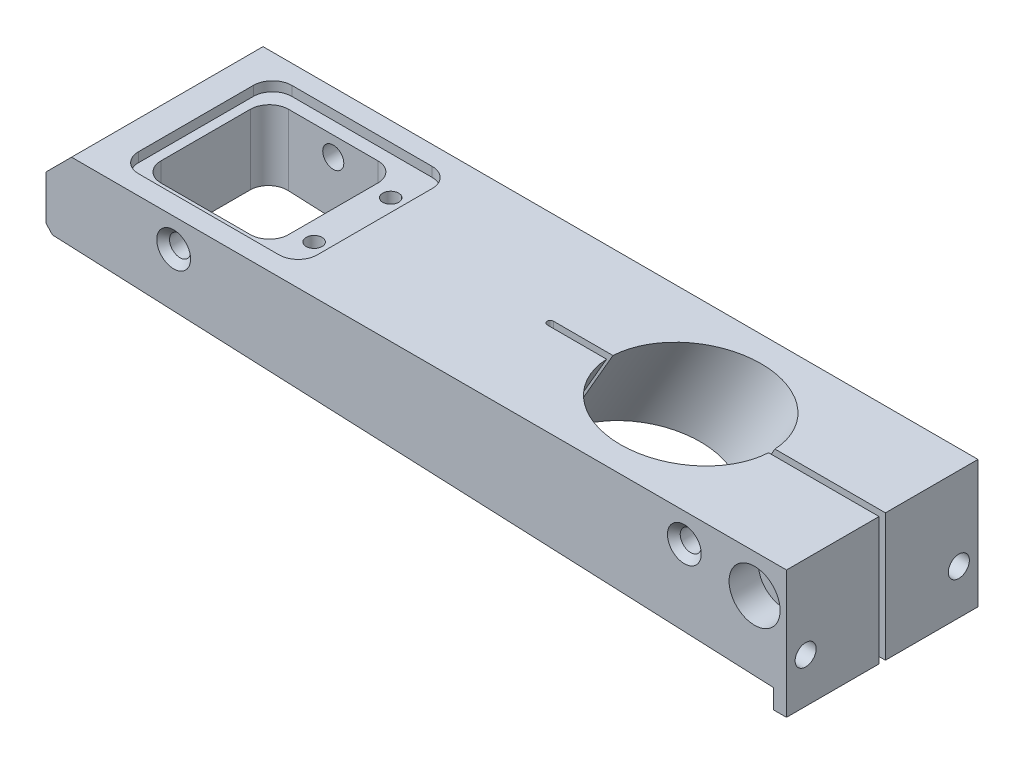
from build123d import *

# Parameters (mm, degrees)
SKETCH1_W                                            = 116
SKETCH1_H                                            = 30
BOSS_EXTRUDE1_DEPTH                                  = 10
CUT_EXTRUDE2_DEPTH                                   = 64.158530699
HOLE_SIZE_PER_SOCKET_HEAD_CAP_SCREW_TYPE_D           = 4.5
HOLE_SIZE_PER_SOCKET_HEAD_CAP_SCREW_TYPE_DEPTH       = 14.5
HOLE_SIZE_PER_SOCKET_HEAD_CAP_SCREW_TYPE_CBORE_D     = 8
HOLE_SIZE_PER_SOCKET_HEAD_CAP_SCREW_TYPE_CBORE_DEPTH = 4.6
M4_TAPPED_HOLE1_D                                    = 3.3
F_5_0_5_DIAMETER_HOLE1_D                             = 5
F_5_0_5_DIAMETER_HOLE1_DEPTH                         = 7
F_5_0_5_DIAMETER_HOLE1_TIP                           = 1.502151548
M4_TAPPED_HOLE2_AT_2_COUNT                           = 2
M4_TAPPED_HOLE2_AT_2_PITCH                           = 80
CHAMFER1_SIZE                                        = 4
M4_TAPPED_HOLE3_D                                    = 3.3
M4_TAPPED_HOLE3_DEPTH                                = 10.1
M4_TAPPED_HOLE3_TIP                                  = 0.991420021
CUT_EXTRUDE3_DEPTH                                   = 67.060578275
SKETCH18_W                                           = 20
SKETCH18_H                                           = 20
CUT_EXTRUDE4_DEPTH                                   = 64.158530699
SKETCH19_W                                           = 28
SKETCH19_H                                           = 24
CUT_EXTRUDE5_DEPTH                                   = 1.5
FILLET1_R                                            = 3
M3_TAPPED_HOLE1_D                                    = 2.5
M3_TAPPED_HOLE1_DEPTH                                = 7.5
M3_TAPPED_HOLE1_TIP                                  = 0.751075774
CHAMFER2_SIZE                                        = 1
CHAMFER2_SIZE2                                       = 1.04665043
CHAMFER3_SIZE                                        = 1


with BuildPart() as part:
    # Sketch1 → Boss-Extrude1 (new, symmetric)
    with BuildSketch(Plane(origin=(0, 0, 0), x_dir=(1, 0, 0), z_dir=(0, 1, 0))):
        Rectangle(SKETCH1_W, SKETCH1_H)
    extrude(amount=BOSS_EXTRUDE1_DEPTH, both=True)

    # Sketch3 → Cut-Revolve1 (revolve, cut)
    with BuildSketch(Plane.XY):
        Polygon((-39.473720558, -128.867912183), (58.526279442, 40.873066959), (49, 46.373066959), (-49, -123.367912183), align=None)
    revolve(axis=Axis((28, 10, 0), (-0.5000000000000041, -0.8660254037844363, 0)), mode=Mode.SUBTRACT)

    # Sketch4 → Cut-Extrude2 (cut, through all)
    with BuildSketch(Plane(origin=(0, 10, 0), x_dir=(1, 0, 0), z_dir=(0, 1, 0))):
        with BuildLine():
            Line((6, 0.5), (58, 0.5))
            Line((58, 0.5), (58, -0.5))
            Line((58, -0.5), (6, -0.5))
            ThreePointArc((6, -0.5), (5.5, 0), (6, 0.5))
        make_face()
    extrude(amount=-CUT_EXTRUDE2_DEPTH, mode=Mode.SUBTRACT)

    # Hole size per socket head cap screw type1
    with Locations(Plane.XY.offset(15)):
        with Locations((53, 4)):
            CounterBoreHole(HOLE_SIZE_PER_SOCKET_HEAD_CAP_SCREW_TYPE_D / 2, HOLE_SIZE_PER_SOCKET_HEAD_CAP_SCREW_TYPE_CBORE_D / 2, HOLE_SIZE_PER_SOCKET_HEAD_CAP_SCREW_TYPE_CBORE_DEPTH, depth=HOLE_SIZE_PER_SOCKET_HEAD_CAP_SCREW_TYPE_DEPTH)

    # M4 Tapped Hole1 (through all)
    with Locations(Plane.XY.offset(-0.5)):
        with Locations((53, 4)):
            Hole(M4_TAPPED_HOLE1_D / 2)

    # Ø5.0 (5) Diameter Hole1
    with Locations(Plane(origin=(0, 0, -15), x_dir=(-1, 0, 0), z_dir=(0, 0, -1))):
        with Locations((-53, 4)):
            Hole(F_5_0_5_DIAMETER_HOLE1_D / 2, depth=F_5_0_5_DIAMETER_HOLE1_DEPTH)
            with Locations((0, 0, -(F_5_0_5_DIAMETER_HOLE1_DEPTH + F_5_0_5_DIAMETER_HOLE1_TIP / 2))):  # 118° drill point
                Cone(0, F_5_0_5_DIAMETER_HOLE1_D / 2, F_5_0_5_DIAMETER_HOLE1_TIP, mode=Mode.SUBTRACT)

    # Sketch11 → M4 Tapped Hole2 (revolve, cut)
    with BuildSketch(Plane(origin=(-38, 5.5, 15), x_dir=(0, -1, 0), z_dir=(1, 0, 0))):
        Polygon((0, 0), (0, 11.091420021), (1.65, 10.1), (1.65, 0), align=None)
    m4_tapped_hole2 = revolve(axis=Axis((-38, 5.5, 21.35), (0, 0, -1)), mode=Mode.SUBTRACT)

    # M4 Tapped Hole2 at 2: M4 Tapped Hole2 ×2
    with Locations(*[(i * M4_TAPPED_HOLE2_AT_2_PITCH, 0, 0) for i in range(1, M4_TAPPED_HOLE2_AT_2_COUNT)]):
        add(m4_tapped_hole2, mode=Mode.SUBTRACT)

    # Mirror1: M4 Tapped Hole2 across plane
    add(m4_tapped_hole2.mirror(Plane.XY), mode=Mode.SUBTRACT)

    # Mirror1 copy 1 sketch → Mirror1 copy 1 (revolve, cut)
    with BuildSketch(Plane(origin=(42, 5.5, -15), x_dir=(0, -1, 0), z_dir=(1, 0, 0))):
        Polygon((0, 0), (0, -11.091420021), (1.65, -10.1), (1.65, 0), align=None)
    revolve(axis=Axis((42, 5.5, -21.35), (0, 0, -1)), mode=Mode.SUBTRACT)

    # Chamfer1
    chamfer1_edges = [part.edges().sort_by_distance(p)[0] for p in [
        (-58, 10, 0),
    ]]
    chamfer(chamfer1_edges, length=CHAMFER1_SIZE)

    # M4 Tapped Hole3
    with Locations(Plane(origin=(58, 0, 0), x_dir=(0, 0, -1), z_dir=(1, 0, 0))):
        with Locations((-12, -3), (12, -3)):
            Hole(M4_TAPPED_HOLE3_D / 2, depth=M4_TAPPED_HOLE3_DEPTH)
            with Locations((0, 0, -(M4_TAPPED_HOLE3_DEPTH + M4_TAPPED_HOLE3_TIP / 2))):  # 118° drill point
                Cone(0, M4_TAPPED_HOLE3_D / 2, M4_TAPPED_HOLE3_TIP, mode=Mode.SUBTRACT)

    # Sketch17 → Cut-Extrude3 (cut, through all)
    with BuildSketch(Plane.XY.offset(15)):
        Polygon((-58, -10), (56, -10), (56, -6.977347492), (-58, -2), align=None)
    extrude(amount=-CUT_EXTRUDE3_DEPTH, mode=Mode.SUBTRACT)

    # Sketch18 → Cut-Extrude4 (cut, through all)
    with BuildSketch(Plane(origin=(0, 10, 0), x_dir=(1, 0, 0), z_dir=(0, 1, 0))):
        with Locations((-38, 0)):
            Rectangle(SKETCH18_W, SKETCH18_H)
    extrude(amount=-CUT_EXTRUDE4_DEPTH, mode=Mode.SUBTRACT)

    # Sketch19 → Cut-Extrude5 (cut)
    with BuildSketch(Plane(origin=(0, 10, 0), x_dir=(1, 0, 0), z_dir=(0, 1, 0))):
        with Locations((-35.5, 0)):
            Rectangle(SKETCH19_W, SKETCH19_H)
    extrude(amount=-CUT_EXTRUDE5_DEPTH, mode=Mode.SUBTRACT)

    # Fillet1
    fillet1_edges = [part.edges().sort_by_distance(p)[0] for p in [
        (-48, 3.031695285, 10),
        (-48, 3.031695285, -10),
        (-28, 2.595085856, -10),
        (-28, 2.595085856, 10),
        (-49.5, 9.25, 12),
        (-49.5, 9.25, -12),
        (-21.5, 9.25, -12),
        (-21.5, 9.25, 12),
    ]]
    fillet(fillet1_edges, radius=FILLET1_R)

    # M3 Tapped Hole1
    with Locations(Plane(origin=(0, 8.5, 0), x_dir=(1, 0, 0), z_dir=(0, 1, 0))):
        with Locations((-25, 6), (-25, -6)):
            Hole(M3_TAPPED_HOLE1_D / 2, depth=M3_TAPPED_HOLE1_DEPTH)
            with Locations((0, 0, -(M3_TAPPED_HOLE1_DEPTH + M3_TAPPED_HOLE1_TIP / 2))):  # 118° drill point
                Cone(0, M3_TAPPED_HOLE1_D / 2, M3_TAPPED_HOLE1_TIP, mode=Mode.SUBTRACT)

    # Chamfer2
    chamfer2_edges = [part.edges().sort_by_distance(p)[0] for p in [
        (-58, -2, 0),
    ]]
    chamfer2_side = [part.faces().sort_by_distance(p)[0] for p in [
        (0.861914044, -4.569966669, 0),
    ]]
    chamfer(chamfer2_edges, length=CHAMFER2_SIZE, length2=CHAMFER2_SIZE2, reference=chamfer2_side[0])

    # Chamfer3
    chamfer3_edges = [part.edges().sort_by_distance(p)[0] for p in [
        (42, 7.15, 15),
        (-38, 7.15, 15),
        (42, 7.15, -15),
        (-38, 7.15, -15),
    ]]
    chamfer(chamfer3_edges, length=CHAMFER3_SIZE)


solid = part.part
